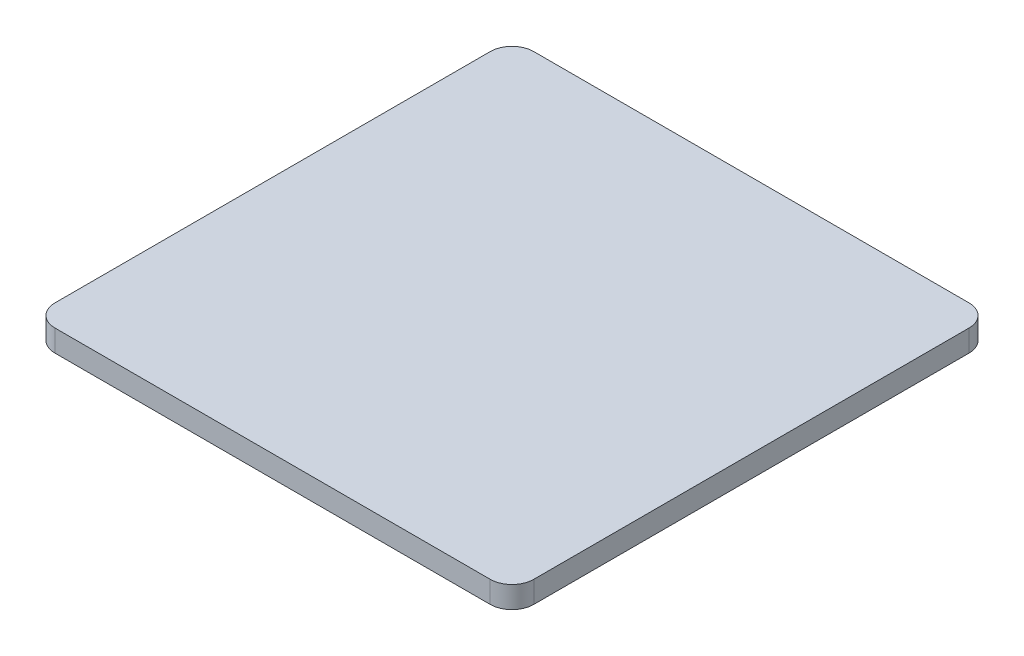
from build123d import *

# Parameters (mm, degrees)
SKETCH_1_W      = 220
SKETCH_1_H      = 220
EXTRUDE_1_DEPTH = 5
FILLET_1_R      = 10


with BuildPart() as part:
    # 草图1 → 凸台-拉伸1 (new, symmetric)
    with BuildSketch(Plane(origin=(0, 0, 0), x_dir=(1, 0, 0), z_dir=(0, 1, 0))):
        Rectangle(SKETCH_1_W, SKETCH_1_H)
    extrude(amount=EXTRUDE_1_DEPTH, both=True)

    # 圆角1
    fillet_1_edges = [part.edges().sort_by_distance(p)[0] for p in [
        (-110, 0, -110),
        (110, 0, -110),
        (110, 0, 110),
        (-110, 0, 110),
    ]]
    fillet(fillet_1_edges, radius=FILLET_1_R)


solid = part.part
